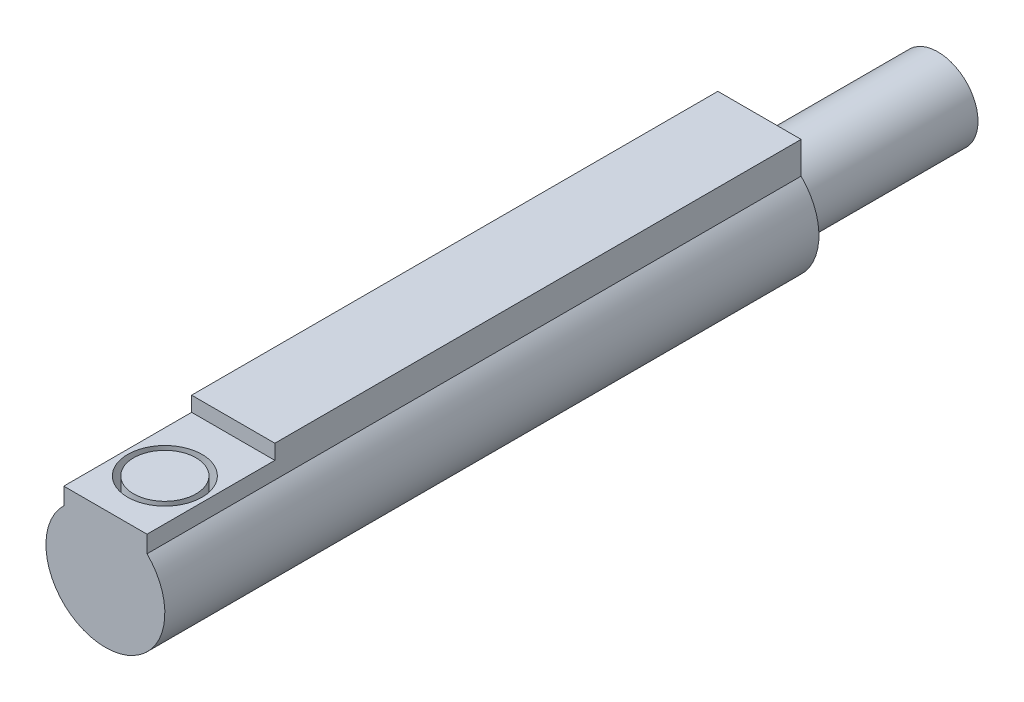
from build123d import *

# Parameters (mm, degrees)
BOSS_EXTRUDE1_DEPTH = 22
SKETCH2_W           = 2.8
SKETCH2_H           = 0.5
BOSS_EXTRUDE2_DEPTH = 17.7
SKETCH3_R           = 1.25
SKETCH3_R_2         = 1.05
CUT_EXTRUDE1_DEPTH  = 1
SKETCH4_R           = 1.35
BOSS_EXTRUDE3_DEPTH = 6


with BuildPart() as part:
    # Sketch1 → Boss-Extrude1 (new body)
    with BuildSketch(Plane.XY):
        with BuildLine():
            Line((1.4, 1.428285686), (1.4, 2))
            Line((1.4, 2), (-1.4, 2))
            Line((-1.4, 2), (-1.4, 1.428285686))
            ThreePointArc((-1.4, 1.428285686), (0, -2), (1.4, 1.428285686))
        make_face()
    extrude(amount=-BOSS_EXTRUDE1_DEPTH)

    # Sketch2 → Boss-Extrude2 (add)
    with BuildSketch(Plane.XY.offset(-22)):
        with Locations((0, 2.25)):
            Rectangle(SKETCH2_W, SKETCH2_H)
    extrude(amount=BOSS_EXTRUDE2_DEPTH)

    # Sketch3 → Cut-Extrude1 (cut)
    with BuildSketch(Plane(origin=(0, 2, 0), x_dir=(1, 0, 0), z_dir=(0, 1, 0))):
        with Locations(Location((0, 2, 0), (0, 0, 270))):
            Circle(SKETCH3_R)
        with Locations(Location((0, 2, 0), (0, 0, 270))):
            Circle(SKETCH3_R_2, mode=Mode.SUBTRACT)
    extrude(amount=-CUT_EXTRUDE1_DEPTH, mode=Mode.SUBTRACT)

    # Sketch4 → Boss-Extrude3 (add)
    with BuildSketch(Plane.XY.offset(-22)):
        Circle(SKETCH4_R)
    extrude(amount=-BOSS_EXTRUDE3_DEPTH)


solid = part.part
